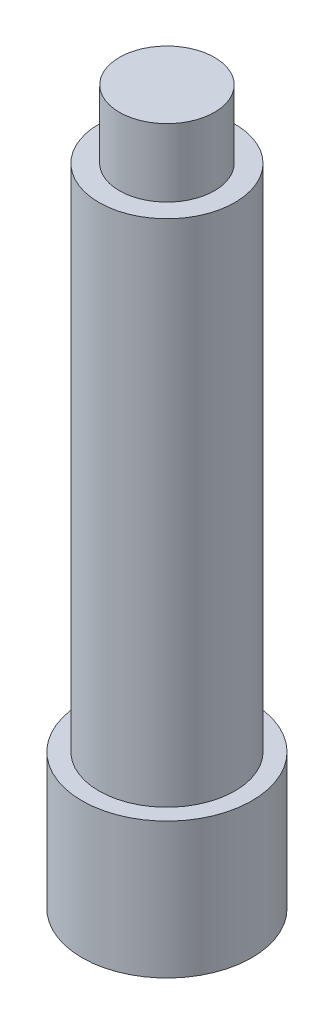
from build123d import *

# Parameters (mm, degrees)
SKETCH1_R           = 12.5
BOSS_EXTRUDE1_DEPTH = 20
SKETCH2_R           = 10
BOSS_EXTRUDE2_DEPTH = 75
SKETCH3_R           = 7
BOSS_EXTRUDE3_DEPTH = 10


with BuildPart() as part:
    # Sketch1 → Boss-Extrude1 (new body)
    with BuildSketch(Plane(origin=(0, 0, 0), x_dir=(1, 0, 0), z_dir=(0, 1, 0))):
        with Locations(Location((0, 0, 0), (0, 0, 270))):
            Circle(SKETCH1_R)
    extrude(amount=BOSS_EXTRUDE1_DEPTH)

    # Sketch2 → Boss-Extrude2 (add)
    with BuildSketch(Plane(origin=(0, 20, 0), x_dir=(1, 0, 0), z_dir=(0, 1, 0))):
        with Locations(Location((0, 0, 0), (0, 0, 270))):
            Circle(SKETCH2_R)
    extrude(amount=BOSS_EXTRUDE2_DEPTH)

    # Sketch3 → Boss-Extrude3 (add)
    with BuildSketch(Plane(origin=(0, 95, 0), x_dir=(1, 0, 0), z_dir=(0, 1, 0))):
        with Locations(Location((0, 0, 0), (0, 0, 270))):
            Circle(SKETCH3_R)
    extrude(amount=BOSS_EXTRUDE3_DEPTH)


solid = part.part
